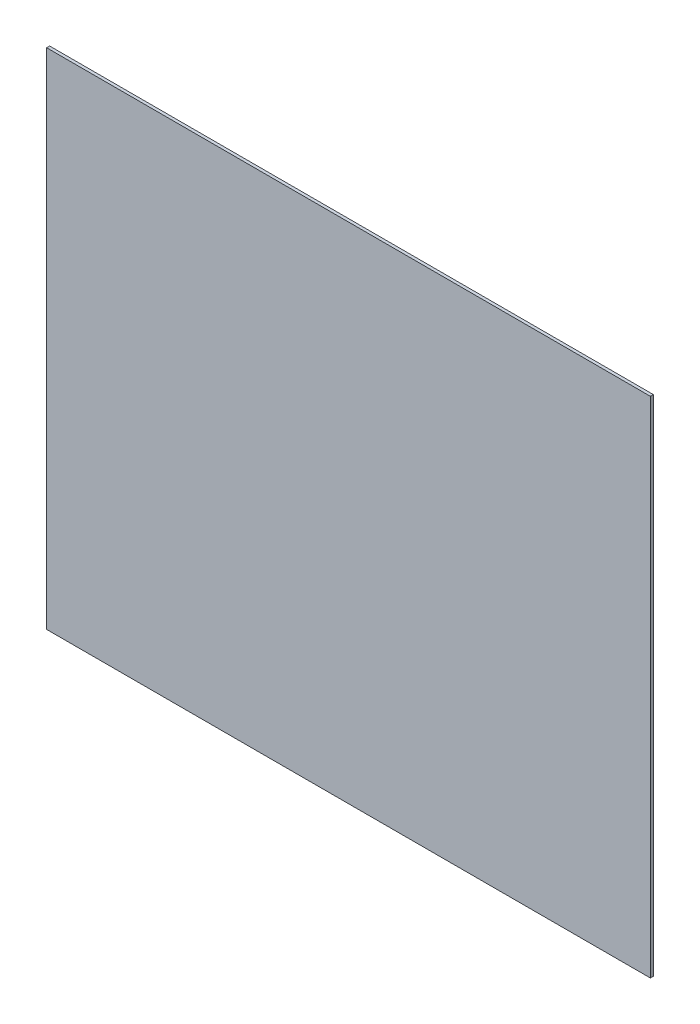
SolidWorks part; units mm, degrees
material "PMMA(有机玻璃)"
ref_plane "前视" through (0, 0, 0) normal (0, 0, 1) x (1, 0, 0)
ref_plane "上视" through (0, 0, 0) normal (0, 1, 0) x (1, 0, 0)
ref_plane "右视" through (0, 0, 0) normal (1, 0, 0) x (0, 0, -1)
sketch "草图1" plane through (0, 0, 0) normal (0, 0, 1) x (1, 0, 0)
  line L1 (-504.5, 421) -> (504.5, 421)
  line L2 (-504.5, 421) -> (-504.5, -421)
  line L3 (-504.5, -421) -> (504.5, -421)
  line L4 (504.5, 421) -> (504.5, -421)
  line L5 (-504.5, 421) -> (504.5, -421) construction
  line L6 (-504.5, -421) -> (504.5, 421) construction
  point P0 (0, 0)
  dimension "D1" = 842
  dimension "D2" = 1009
extrude "凸台-拉伸1" add sketch "草图1" along normal blind 5
hole_wizard "M5 间隙孔1" positions "草图3" profile "草图2" hole size "M5" standard "GB"
sketch "草图3" plane through (0, 0, 5) normal (0, 0, 1) x (1, 0, 0)
  line L0 (-427.5, 273) -> (-427.5, -273) construction
  line L1 (-427.5, -273) -> (427.5, -273) construction
  line L2 (0, 273) -> (0, -273) construction
  line L3 (427.5, 273) -> (-427.5, 273) construction
  line L5 (-427.5, 0) -> (427.5, 0) construction
  line L6 (427.5, -273) -> (427.5, 273) construction
  point P0 (-375, -261)
  point P46 (415.5, 250)
  point P48 (-415.5, 250)
  point P58 (-125, -261)
  point P59 (125, -261)
  point P61 (-125, 261)
  point P62 (125, 261)
  point P64 (-375, 261)
  point P88 (375, -261)
  point P89 (375, 261)
  point P108 (415.5, 0)
  point P109 (-415.5, 0)
  point P110 (415.5, -250)
  point P111 (-415.5, -250)
  dimension "D1" = 12
  dimension "D2" = 12
  dimension "D5" = 3
  dimension "D3" = 12
  dimension "D6" = 4
  dimension "D4" = 2
sketch "草图2" plane through (-375, -261, 5) normal (1, 0, 0) x (0, -1, 0)
  line L0 (0, 0) -> (0, 5)
  line L1 (0, 5) -> (2.75, 5)
  line L2 (2.75, 5) -> (2.75, 0)
  line L5 (2.75, 0) -> (0, 0)
  line L11 (0, -6.35) -> (0, 107.95) construction
  dimension "通孔孔直径" = 5.5
  dimension "通孔孔深度" = 5
